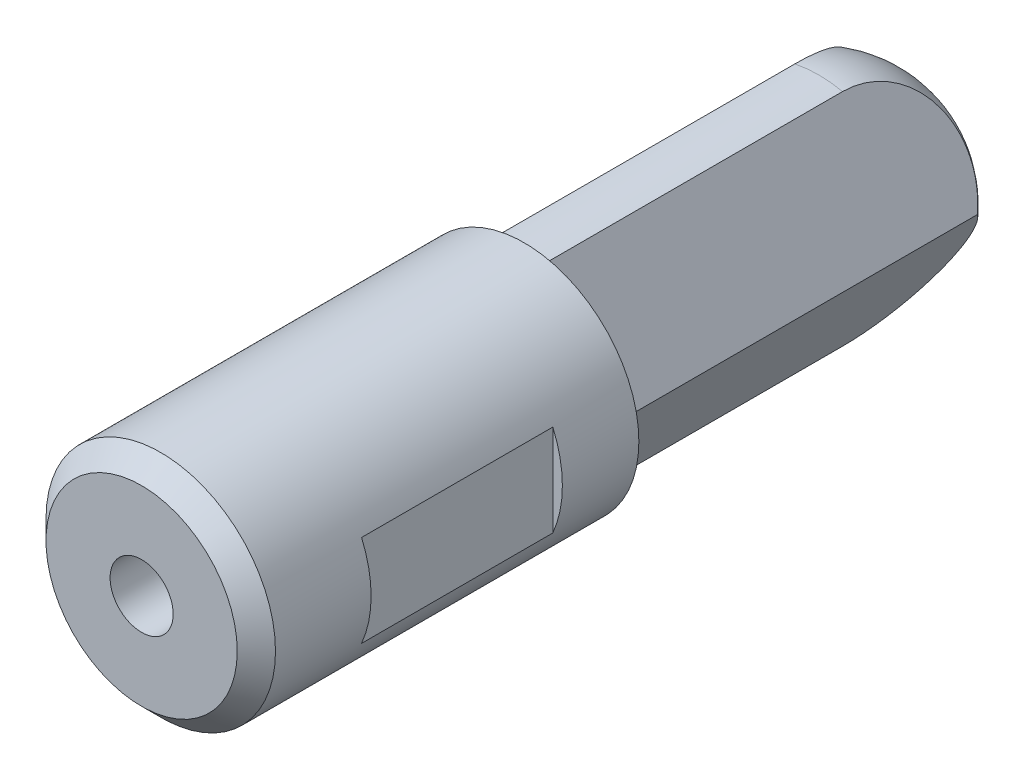
SolidWorks part; units mm, degrees
material "AISI 304"
ref_plane "Front Plane" through (0, 0, 0) normal (0, 0, 1) x (1, 0, 0)
ref_plane "Top Plane" through (0, 0, 0) normal (0, 1, 0) x (1, 0, 0)
ref_plane "Right Plane" through (0, 0, 0) normal (1, 0, 0) x (0, 0, -1)
sketch "Sketch1" plane through (0, 0, 0) normal (0, 0, 1) x (1, 0, 0)
  circle A0 centre (0, 0) radius 5.9
  dimension "D1" = 11.8
extrude "Boss-Extrude1" add sketch "Sketch1" along normal blind 35.4
sketch "Sketch2" plane through (0, 0, 0) normal (0, 1, 0) x (1, 0, 0)
  line L0 (0, 5.9) -> (0, 0)
  line L1 (0, 0) -> (-5.9, 0)
  arc A0 (0, 5.9) -> (-5.9, 0) centre (0, 0) ccw
  dimension "D1" = 11.8
revolve "Revolve1" add sketch "Sketch2" angle 360 about L0
hole_wizard "M4 Tapped Hole1" positions "Sketch3" profile "Sketch4" tap size "M4" standard "GB"
sketch "Sketch3" plane through (0, 0, 35.4) normal (0, 0, 1) x (1, 0, 0)
  point P0 (0, 0)
sketch "Sketch4" plane through (0, 0, 35.4) normal (1, 0, 0) x (0, -1, 0)
  line L0 (0, 0) -> (0, 11.0914)
  line L1 (0, 11.0914) -> (1.65, 10.1)
  line L2 (1.65, 10.1) -> (1.65, 0)
  line L5 (1.65, 0) -> (0, 0)
  line L10 (0, 11.0914) -> (-1.65, 10.1) construction
  line L11 (0, -6.35) -> (0, 107.95) construction
  dimension "螺纹孔钻头直径" = 3.3
  dimension "螺纹孔钻头深度" = 10.1
  dimension "导头角度" = 118
cosmetic thread "Cosmetic thread 1"
sketch "Sketch5" plane through (0, 0, 35.4) normal (0, 0, 1) x (1, 0, 0)
  circle A0 centre (0, 0) radius 6
  circle A1 centre (0, 0) radius 4
  dimension "D1" = 12
  dimension "D2" = 8
extrude "Boss-Extrude2" add sketch "Sketch5" against normal blind 20
chamfer "Chamfer1" distance 1 angle 45 1 edges at (6, 0, 35.4)
sketch "Sketch6" plane through (0, 0, 0) normal (0, 1, 0) x (1, 0, 0)
  line L0 (-5, -35.4) -> (5, -35.4) construction
  line L1 (-7.5263, -19.4) -> (-5.5, -19.4)
  line L2 (-7.5263, -19.4) -> (-7.5263, -29.4)
  line L3 (-7.5263, -29.4) -> (-5.5, -29.4)
  line L4 (-5.5, -19.4) -> (-5.5, -29.4)
  line L5 (7.5263, -19.4) -> (5.5, -19.4)
  line L6 (7.5263, -19.4) -> (7.5263, -29.4)
  line L7 (7.5263, -29.4) -> (5.5, -29.4)
  line L8 (5.5, -19.4) -> (5.5, -29.4)
  line L9 (0, -35.4) -> (0, -40.7235) construction
  dimension "D1" = 11
  dimension "D2" = 6
  dimension "D3" = 10
extrude "Cut-Extrude1" cut sketch "Sketch6" against normal through all both and the other way through all
sketch "Sketch7" plane through (0, 0, 15.4) normal (0, 0, -1) x (-1, 0, 0)
  line L0 (-1.25, 5.7661) -> (-4.579, 0)
  line L1 (-4.579, 0) -> (-1.25, -5.7661)
  line L2 (0, 0) -> (0, 2.7292) construction
  line L3 (4.579, 0) -> (1.25, -5.7661)
  line L4 (1.25, 5.7661) -> (4.579, 0)
  arc A0 (-1.25, -5.7661) -> (1.25, -5.7661) centre (0, 0) ccw
  arc A2 (1.25, 5.7661) -> (-1.25, 5.7661) centre (0, 0) ccw
  dimension "D1" = 11.8
  dimension "D2" = 30
  dimension "D3" = 1.25
extrude "Cut-Extrude2" cut sketch "Sketch7" along normal through all flip side to cut
